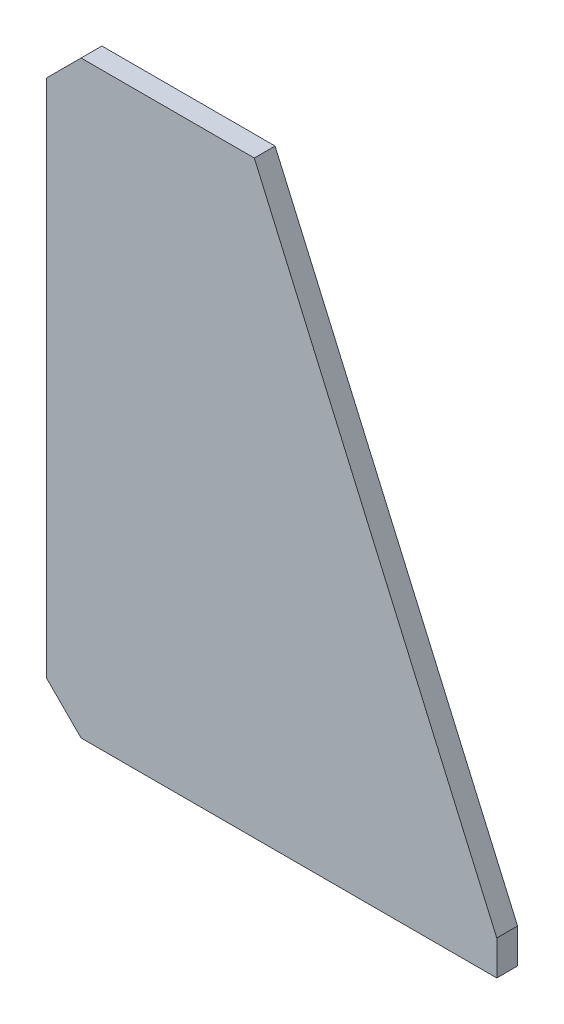
SolidWorks part; units mm, degrees
material "Q235B"
ref_plane "Front Plane" through (0, 0, 0) normal (0, 0, 1) x (1, 0, 0)
ref_plane "Top Plane" through (0, 0, 0) normal (0, 1, 0) x (1, 0, 0)
ref_plane "Right Plane" through (0, 0, 0) normal (1, 0, 0) x (0, 0, -1)
sketch "Sketch1" plane through (0, 0, 0) normal (0, 0, 1) x (1, 0, 0)
  line L0 (0, 170) -> (0, 0)
  line L1 (0, 0) -> (130, 0)
  line L2 (130, 0) -> (130, 10)
  line L3 (130, 10) -> (60, 170)
  line L4 (60, 170) -> (0, 170)
  dimension "D1" = 130
  dimension "D2" = 10
  dimension "D3" = 170
  dimension "D4" = 60
extrude "Boss-Extrude1" add sketch "Sketch1" along normal mid plane 6
chamfer "Chamfer1" distance 10 angle 45 2 edges at (0, 0, 0) (0, 170, 0)
